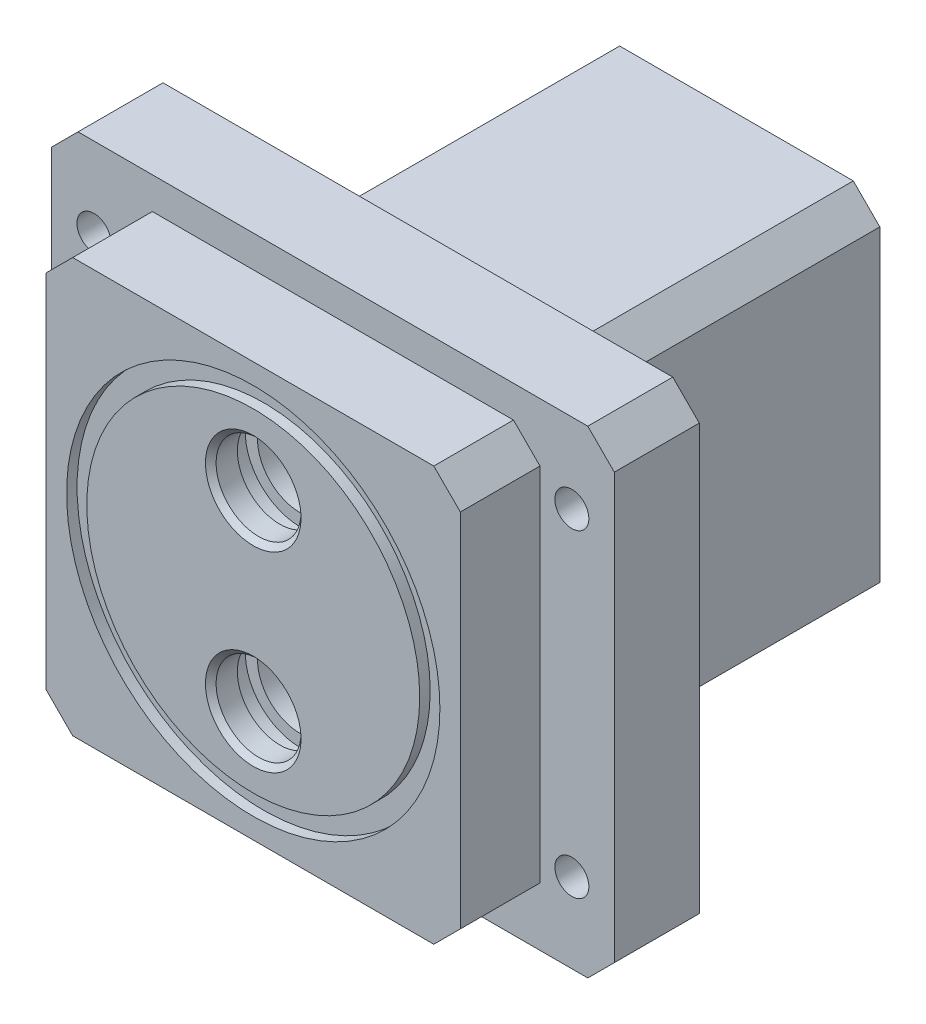
SolidWorks part; units mm, degrees
material "Q235-A"
ref_plane "Front Plane" through (0, 0, 0) normal (0, 0, 1) x (1, 0, 0)
ref_plane "Top Plane" through (0, 0, 0) normal (0, 1, 0) x (1, 0, 0)
ref_plane "Right Plane" through (0, 0, 0) normal (1, 0, 0) x (0, 0, -1)
sketch "Sketch1" plane through (0, 0, 0) normal (0, 0, 1) x (1, 0, 0)
  line L1 (-27, -34) -> (27, -34)
  line L2 (-27, -34) -> (-27, 34)
  line L3 (-27, 34) -> (27, 34)
  line L4 (27, -34) -> (27, 34)
  line L5 (-27, -34) -> (27, 34) construction
  line L6 (-27, 34) -> (27, -34) construction
  point P0 (0, 0)
  dimension "D1" = 54
  dimension "D2" = 68
extrude "Boss-Extrude1" add sketch "Sketch1" along normal blind 60
sketch "Sketch2" plane through (0, 0, 60) normal (0, 0, 1) x (1, 0, 0)
  line L1 (53, 45) -> (-53, 45)
  line L2 (53, 45) -> (53, -45)
  line L3 (53, -45) -> (-53, -45)
  line L4 (-53, 45) -> (-53, -45)
  line L5 (53, 45) -> (-53, -45) construction
  line L6 (53, -45) -> (-53, 45) construction
  point P0 (0, 0)
  dimension "D1" = 106
  dimension "D2" = 90
extrude "Boss-Extrude2" add sketch "Sketch2" along normal blind 16
sketch "Sketch3" plane through (0, 0, 76) normal (0, 0, 1) x (1, 0, 0)
  line L1 (39, 39) -> (-39, 39)
  line L2 (39, 39) -> (39, -39)
  line L3 (39, -39) -> (-39, -39)
  line L4 (-39, 39) -> (-39, -39)
  line L5 (39, 39) -> (-39, -39) construction
  line L6 (39, -39) -> (-39, 39) construction
  point P0 (0, 0)
  dimension "D1" = 78
  dimension "D2" = 78
extrude "Boss-Extrude3" add sketch "Sketch3" along normal blind 15
chamfer "Chamfer1" distance 5 angle 45 12 edges at (-27, 34, 30) (-53, 45, 68) (-39, 39, 83.5) (-53, -45, 68) (-27, -34, 30) (-39, -39, 83.5) (39, -39, 83.5) (39, 39, 83.5) (53, 45, 68) (53, -45, 68) (27, 34, 30) (27, -34, 30)
sketch "Sketch4" plane through (0, 0, 91) normal (0, 0, 1) x (1, 0, 0)
  circle A0 centre (0, 0) radius 35.15
  circle A1 centre (0, 0) radius 31.35
extrude "Cut-Extrude1" cut sketch "Sketch4" against normal blind 1.97
sketch "Sketch5" plane through (0, 0, 91) normal (0, 0, 1) x (1, 0, 0)
  line L0 (0, 18) -> (0, -18)
  point P5 (0, 0)
hole_wizard "Hole1" positions "Sketch6" profile "Sketch7" legacy end condition through all
sketch "Sketch6" plane through (0, 0, 91) normal (0, 0, 1) x (1, 0, 0)
  point P0 (0, -18)
  point P3 (0, 18)
sketch "Sketch7" plane through (0, -18, 91) normal (1, 0, 0) x (0, -1, 0)
  line L0 (0, 0) -> (0, 91)
  line L1 (0, 91) -> (8, 91)
  line L2 (8, 91) -> (8, 0)
  line L3 (8, 0) -> (0, 0)
  line L4 (0, 110) -> (0, -10) construction
  dimension "直径" = 16
  dimension "深度" = 91
hole_wizard "Hole2" positions "Sketch8" profile "Sketch9" legacy
sketch "Sketch8" plane through (0, 0, 0) normal (0, 0, -1) x (-1, 0, 0)
  point P0 (0, 18)
  point P3 (0, -18)
sketch "Sketch9" plane through (0, 18, 0) normal (1, 0, 0) x (0, 1, 0)
  line L0 (0, 0) -> (0, 63)
  line L1 (0, 63) -> (11, 63)
  line L2 (11, 63) -> (11, 0)
  line L3 (11, 0) -> (0, 0)
  line L4 (0, 110) -> (0, -10) construction
  dimension "直径" = 22
  dimension "深度" = 63
chamfer "Chamfer2" distance 1 angle 45 4 edges at (8, -18, 91) (8, 18, 91) (-11, 18, 0) (-11, -18, 0)
sketch "Sketch10" plane through (0, 0, 0) normal (0, 0, -1) x (-1, 0, 0)
  line L1 (20, 18) -> (-20, 18)
  line L2 (20, 18) -> (20, -18)
  line L3 (20, -18) -> (-20, -18)
  line L4 (-20, 18) -> (-20, -18)
  line L5 (20, 18) -> (-20, -18) construction
  line L6 (20, -18) -> (-20, 18) construction
  point P0 (0, 0)
  dimension "D1" = 36
  dimension "D2" = 40
hole_wizard "M5 Tapped Hole1" positions "Sketch11" profile "Sketch12" tap size "M5" standard "GB"
sketch "Sketch11" plane through (0, 0, 0) normal (0, 0, -1) x (-1, 0, 0)
  point P0 (20, -18)
  point P3 (20, 18)
  point P6 (-20, 18)
  point P9 (-20, -18)
sketch "Sketch12" plane through (-20, -18, 0) normal (1, 0, 0) x (0, 1, 0)
  line L0 (0, 0) -> (0, 11.2618)
  line L1 (0, 11.2618) -> (2.1, 10)
  line L2 (2.1, 10) -> (2.1, 0)
  line L5 (2.1, 0) -> (0, 0)
  line L10 (0, 11.2618) -> (-2.1, 10) construction
  line L11 (0, -6.35) -> (0, 107.95) construction
  dimension "螺纹孔钻头直径" = 4.2
  dimension "螺纹孔钻头深度" = 10
  dimension "导头角度" = 118
cosmetic thread "Cosmetic Thread1" parameters "D1"=10, "D2"=5
cosmetic thread "Cosmetic Thread2" parameters "D1"=10, "D2"=5
cosmetic thread "Cosmetic Thread3" parameters "D1"=10, "D2"=5
cosmetic thread "Cosmetic Thread4" parameters "D1"=10, "D2"=5
sketch "Sketch13" plane through (0, 0, 60) normal (0, 0, -1) x (-1, 0, 0)
  line L1 (45, 30) -> (-45, 30)
  line L2 (45, 30) -> (45, -30)
  line L3 (45, -30) -> (-45, -30)
  line L4 (-45, 30) -> (-45, -30)
  line L5 (45, 30) -> (-45, -30) construction
  line L6 (45, -30) -> (-45, 30) construction
  point P0 (0, 0)
  dimension "D1" = 60
  dimension "D2" = 90
hole_wizard "Hole3" positions "Sketch14" profile "Sketch15" legacy end condition through all
sketch "Sketch14" plane through (0, 0, 60) normal (0, 0, -1) x (-1, 0, 0)
  point P0 (45, -30)
  point P3 (45, 30)
  point P6 (-45, 30)
  point P9 (-45, -30)
sketch "Sketch15" plane through (-45, -30, 60) normal (1, 0, 0) x (0, 1, 0)
  line L0 (0, 0) -> (0, 31)
  line L1 (0, 31) -> (3.2, 31)
  line L2 (3.2, 31) -> (3.2, 9)
  line L3 (3.2, 9) -> (5.5, 9)
  line L4 (5.5, 9) -> (5.5, 0)
  line L5 (5.5, 0) -> (0, 0)
  line L6 (0, 110) -> (0, -10) construction
  dimension "直径" = 6.4
  dimension "深度" = 31
  dimension "柱坑直径" = 11
  dimension "柱坑深度" = 9
ref_plane "Plane1" through (0, 0, 86) normal (0, 0, 1) x (1, 0, 0)
sketch "Sketch16" plane through (0, 0, 86) normal (0, 0, 1) x (1, 0, 0)
  circle A0 centre (0, 18) radius 10.3
  circle A1 centre (0, -18) radius 10.3
extrude "Cut-Extrude2" cut sketch "Sketch16" against normal blind 3.8
